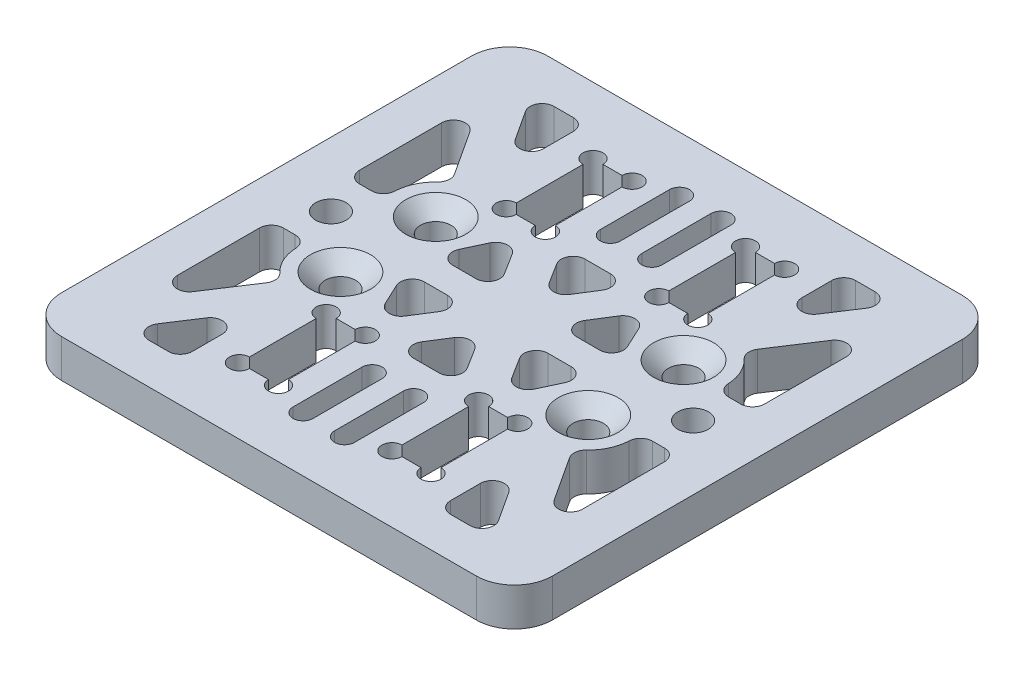
from build123d import *

# Parameters (mm, degrees)
SKETCH_1_W                   = 51.5
SKETCH_1_H                   = 51
SKETCH_1_R                   = 1.6
EXTRUDE_1_DEPTH              = 4
HOLE_WIZARD_M3_1_D           = 3.2
HOLE_WIZARD_M3_1_DEPTH       = 3.03862301
HOLE_WIZARD_M3_1_CSINK_D     = 6.3
HOLE_WIZARD_M3_1_CSINK_ANGLE = 90
HOLE_WIZARD_M3_1_TIP         = 0.96137699
CUT_EXTRUDE_2_DEPTH          = 37.459738068
FILLET_R1_25_R               = 1.25
FILLET_R4_R                  = 4


with BuildPart() as part:
    # 草图1 → 凸台-拉伸1 (new body)
    with BuildSketch(Plane(origin=(0, 0, 0), x_dir=(1, 0, 0), z_dir=(0, 1, 0))):
        Rectangle(SKETCH_1_W, SKETCH_1_H)
        with Locations(Location((-19, 0, 0), (0, 0, 270))):
            Circle(SKETCH_1_R, mode=Mode.SUBTRACT)
        with Locations(Location((19, 0, 0), (0, 0, 90))):
            Circle(SKETCH_1_R, mode=Mode.SUBTRACT)
        with Locations(Location((-13, 5, 0), (0, 0, 270))):
            Circle(SKETCH_1_R, mode=Mode.SUBTRACT)
        with Locations(Location((-13, -5, 0), (0, 0, 270))):
            Circle(SKETCH_1_R, mode=Mode.SUBTRACT)
        with Locations(Location((13, -5, 0), (0, 0, 90))):
            Circle(SKETCH_1_R, mode=Mode.SUBTRACT)
        with Locations(Location((13, 5, 0), (0, 0, 90))):
            Circle(SKETCH_1_R, mode=Mode.SUBTRACT)
        with BuildLine():
            Line((7, 9.45), (9, 9.45))
            ThreePointArc((9, 9.45), (10.79246212, 8.70753788), (10.05, 10.5))
            Line((10.05, 10.5), (10.05, 17.5))
            ThreePointArc((10.05, 17.5), (10.79246212, 19.29246212), (9, 18.55))
            Line((9, 18.55), (7, 18.55))
            ThreePointArc((7, 18.55), (5.20753788, 19.29246212), (5.95, 17.5))
            Line((5.95, 17.5), (5.95, 10.5))
            ThreePointArc((5.95, 10.5), (5.20753788, 8.70753788), (7, 9.45))
        make_face(mode=Mode.SUBTRACT)
        with BuildLine():
            Line((-7, 9.45), (-9, 9.45))
            ThreePointArc((-9, 9.45), (-10.79246212, 8.70753788), (-10.05, 10.5))
            Line((-10.05, 10.5), (-10.05, 17.5))
            ThreePointArc((-10.05, 17.5), (-10.79246212, 19.29246212), (-9, 18.55))
            Line((-9, 18.55), (-7, 18.55))
            ThreePointArc((-7, 18.55), (-5.20753788, 19.29246212), (-5.95, 17.5))
            Line((-5.95, 17.5), (-5.95, 10.5))
            ThreePointArc((-5.95, 10.5), (-5.20753788, 8.70753788), (-7, 9.45))
        make_face(mode=Mode.SUBTRACT)
        with BuildLine():
            Line((10.05, -10.5), (10.05, -17.5))
            ThreePointArc((10.05, -17.5), (10.79246212, -19.29246212), (9, -18.55))
            Line((9, -18.55), (7, -18.55))
            ThreePointArc((7, -18.55), (5.20753788, -19.29246212), (5.95, -17.5))
            Line((5.95, -17.5), (5.95, -10.5))
            ThreePointArc((5.95, -10.5), (5.20753788, -8.70753788), (7, -9.45))
            Line((7, -9.45), (9, -9.45))
            ThreePointArc((9, -9.45), (10.79246212, -8.70753788), (10.05, -10.5))
        make_face(mode=Mode.SUBTRACT)
        with BuildLine():
            Line((-7, -9.45), (-9, -9.45))
            ThreePointArc((-9, -9.45), (-10.79246212, -8.70753788), (-10.05, -10.5))
            Line((-10.05, -10.5), (-10.05, -17.5))
            ThreePointArc((-10.05, -17.5), (-10.79246212, -19.29246212), (-9, -18.55))
            Line((-9, -18.55), (-7, -18.55))
            ThreePointArc((-7, -18.55), (-5.20753788, -19.29246212), (-5.95, -17.5))
            Line((-5.95, -17.5), (-5.95, -10.5))
            ThreePointArc((-5.95, -10.5), (-5.20753788, -8.70753788), (-7, -9.45))
        make_face(mode=Mode.SUBTRACT)
    extrude(amount=EXTRUDE_1_DEPTH)

    # M3 锥形沉头孔1
    with Locations(Plane(origin=(0, 4, 0), x_dir=(1, 0, 0), z_dir=(0, 1, 0))):
        with Locations((-13, 5), (13, 5), (-13, -5), (13, -5)):
            CounterSinkHole(HOLE_WIZARD_M3_1_D / 2, HOLE_WIZARD_M3_1_CSINK_D / 2, depth=HOLE_WIZARD_M3_1_DEPTH, counter_sink_angle=HOLE_WIZARD_M3_1_CSINK_ANGLE)
            with Locations((0, 0, -(HOLE_WIZARD_M3_1_DEPTH + HOLE_WIZARD_M3_1_TIP / 2))):  # 118° drill point
                Cone(0, HOLE_WIZARD_M3_1_D / 2, HOLE_WIZARD_M3_1_TIP, mode=Mode.SUBTRACT)

    # 草图7 → 切除-拉伸2 (cut, through all)
    with BuildSketch(Plane(origin=(0, 4, 0), x_dir=(1, 0, 0), z_dir=(0, 1, 0))):
        Polygon((-13.55, 21.25), (-19.159509695, 21.25), (-13.55, 12.665455817), align=None)
        with BuildLine():
            Line((-15.263478993, 8.889301074), (-21.25, 18.050806602))
            Line((-21.25, 18.050806602), (-21.25, 4))
            Line((-21.25, 4), (-17.387482194, 4))
            ThreePointArc((-17.387482194, 4), (-17.127364465, 6.793003785), (-15.263478993, 8.889301074))
        make_face()
        with BuildLine():
            Line((-3.225, 19.75), (-3.225, 12.5))
            ThreePointArc((-3.225, 12.5), (-2.175, 11.45), (-1.125, 12.5))
            Line((-1.125, 12.5), (-1.125, 19.75))
            ThreePointArc((-1.125, 19.75), (-2.175, 20.8), (-3.225, 19.75))
        make_face()
        with BuildLine():
            ThreePointArc((3.225, 12.5), (2.175, 11.45), (1.125, 12.5))
            Line((1.125, 12.5), (1.125, 19.75))
            ThreePointArc((1.125, 19.75), (2.175, 20.8), (3.225, 19.75))
            Line((3.225, 19.75), (3.225, 12.5))
        make_face()
        Polygon((13.55, 12.665455817), (19.159509695, 21.25), (13.55, 21.25), align=None)
        with BuildLine():
            Line((21.25, 4), (21.25, 18.050806602))
            Line((21.25, 18.050806602), (15.263478993, 8.889301074))
            ThreePointArc((15.263478993, 8.889301074), (17.127364465, 6.793003785), (17.387482194, 4))
            Line((17.387482194, 4), (21.25, 4))
        make_face()
        Polygon((3.598677909, 9), (-3.598677909, 9), (0, 3.284452733), align=None)
        Polygon((3.598677909, -9), (0, -3.284452733), (-3.598677909, -9), align=None)
        with BuildLine():
            Line((-21.25, -4), (-21.25, -18.050806602))
            Line((-21.25, -18.050806602), (-15.263478993, -8.889301074))
            ThreePointArc((-15.263478993, -8.889301074), (-17.127364465, -6.793003785), (-17.387482194, -4))
            Line((-17.387482194, -4), (-21.25, -4))
        make_face()
        Polygon((-13.55, -12.665455817), (-19.159509695, -21.25), (-13.55, -21.25), align=None)
        with BuildLine():
            ThreePointArc((-3.225, -12.5), (-2.175, -11.45), (-1.125, -12.5))
            Line((-1.125, -12.5), (-1.125, -19.75))
            ThreePointArc((-1.125, -19.75), (-2.175, -20.8), (-3.225, -19.75))
            Line((-3.225, -19.75), (-3.225, -12.5))
        make_face()
        with BuildLine():
            Line((3.225, -19.75), (3.225, -12.5))
            ThreePointArc((3.225, -12.5), (2.175, -11.45), (1.125, -12.5))
            Line((1.125, -12.5), (1.125, -19.75))
            ThreePointArc((1.125, -19.75), (2.175, -20.8), (3.225, -19.75))
        make_face()
        Polygon((13.55, -21.25), (19.159509695, -21.25), (13.55, -12.665455817), align=None)
        with BuildLine():
            Line((15.263478993, -8.889301074), (21.25, -18.050806602))
            Line((21.25, -18.050806602), (21.25, -4))
            Line((21.25, -4), (17.387482194, -4))
            ThreePointArc((17.387482194, -4), (17.127364465, -6.793003785), (15.263478993, -8.889301074))
        make_face()
        Polygon((-3.012433202, 1.5), (-6.831561162, 7.565673817), (-9.669319563, 1.5), align=None)
        Polygon((6.831561162, 7.565673817), (3.012433202, 1.5), (9.669319563, 1.5), align=None)
        Polygon((-6.831561162, -7.565673817), (-3.012433202, -1.5), (-9.669319563, -1.5), align=None)
        Polygon((9.669319563, -1.5), (3.012433202, -1.5), (6.831561162, -7.565673817), align=None)
    extrude(amount=-CUT_EXTRUDE_2_DEPTH, mode=Mode.SUBTRACT)

    # R1.25 镂空圆角
    fillet_r1_25_edges = [part.edges().sort_by_distance(p)[0] for p in [
        (-19.159509695, 2, 21.25),
        (-13.55, 2, 12.665455817),
        (-13.55, 2, 21.25),
        (13.55, 2, 21.25),
        (13.55, 2, 12.665455817),
        (19.159509695, 2, 21.25),
        (-9.669319563, 2, 1.5),
        (-3.012433202, 2, 1.5),
        (-6.831561162, 2, 7.565673817),
        (3.012433202, 2, -1.5),
        (6.831561162, 2, -7.565673817),
        (9.669319563, 2, -1.5),
        (-9.669319563, 2, -1.5),
        (-6.831561162, 2, -7.565673817),
        (-3.012433202, 2, -1.5),
        (15.263478993, 2, 8.889301074),
        (17.387482194, 2, 4),
        (21.25, 2, 4),
        (21.25, 2, 18.050806602),
        (-15.263478993, 2, -8.889301074),
        (-17.387482194, 2, -4),
        (-21.25, 2, -4),
        (-21.25, 2, -18.050806602),
        (19.159509695, 2, -21.25),
        (13.55, 2, -12.665455817),
        (13.55, 2, -21.25),
        (15.263478993, 2, -8.889301074),
        (21.25, 2, -18.050806602),
        (21.25, 2, -4),
        (17.387482194, 2, -4),
        (-3.598677909, 2, -9),
        (3.598677909, 2, -9),
        (0, 2, -3.284452733),
        (-3.598677909, 2, 9),
        (0, 2, 3.284452733),
        (3.598677909, 2, 9),
        (-15.263478993, 2, 8.889301074),
        (-21.25, 2, 18.050806602),
        (-21.25, 2, 4),
        (-17.387482194, 2, 4),
        (3.012433202, 2, 1.5),
        (9.669319563, 2, 1.5),
        (6.831561162, 2, 7.565673817),
        (-19.159509695, 2, -21.25),
        (-13.55, 2, -21.25),
        (-13.55, 2, -12.665455817),
    ]]
    fillet(fillet_r1_25_edges, radius=FILLET_R1_25_R)

    # R4 外缘圆角
    fillet_r4_edges = [part.edges().sort_by_distance(p)[0] for p in [
        (25.75, 2, 25.5),
        (-25.75, 2, 25.5),
        (-25.75, 2, -25.5),
        (25.75, 2, -25.5),
    ]]
    fillet(fillet_r4_edges, radius=FILLET_R4_R)


solid = part.part
